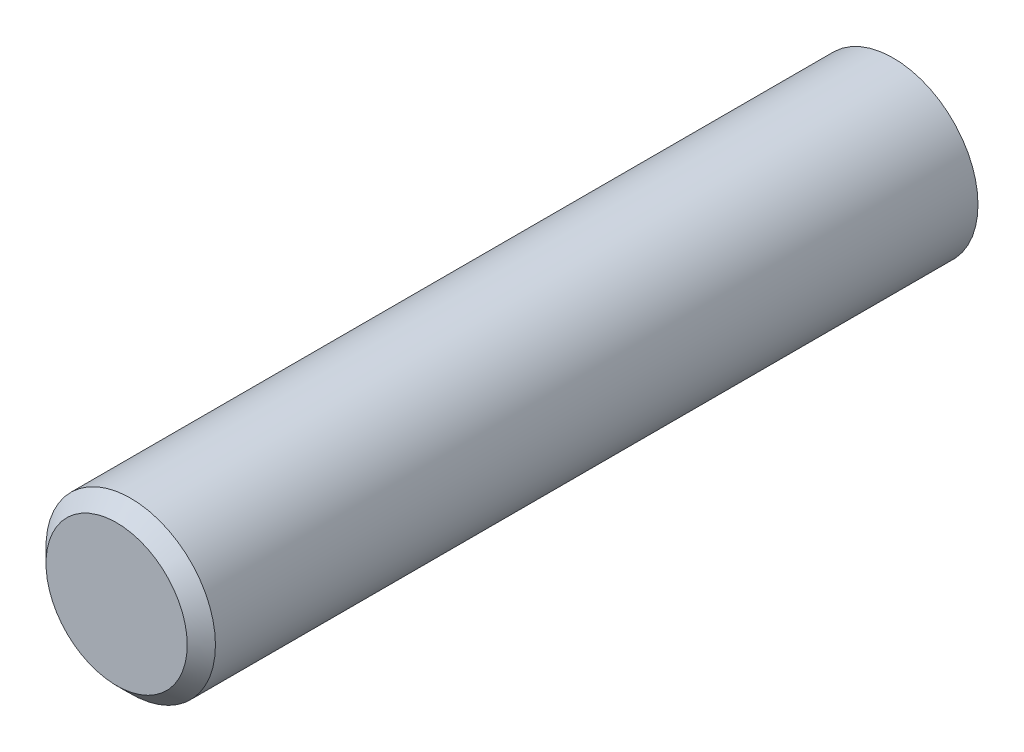
SolidWorks part; units mm, degrees
ref_plane "Front" through (0, 0, 0) normal (0, 0, 1) x (1, 0, 0)
ref_plane "Top" through (0, 0, 0) normal (0, 1, 0) x (1, 0, 0)
ref_plane "Right" through (0, 0, 0) normal (1, 0, 0) x (0, 0, -1)
sketch "Sketch1" plane through (0, 0, 0) normal (0, 0, 1) x (1, 0, 0)
  circle A0 centre (0, 0) radius 6
extrude "Boss-Extrude1" add sketch "Sketch1" along normal blind 55
cosmetic thread "Cosmetic Thread1" parameters "D2"=10.106
chamfer "Chamfer1" distance 1 angle 45 1 edges at (6, 0, 55)
sketch "Sketch2" plane through (0, 0, 55) normal (0, 0, 1) x (1, 0, 0)
  circle A0 centre (0, 0) radius 6
